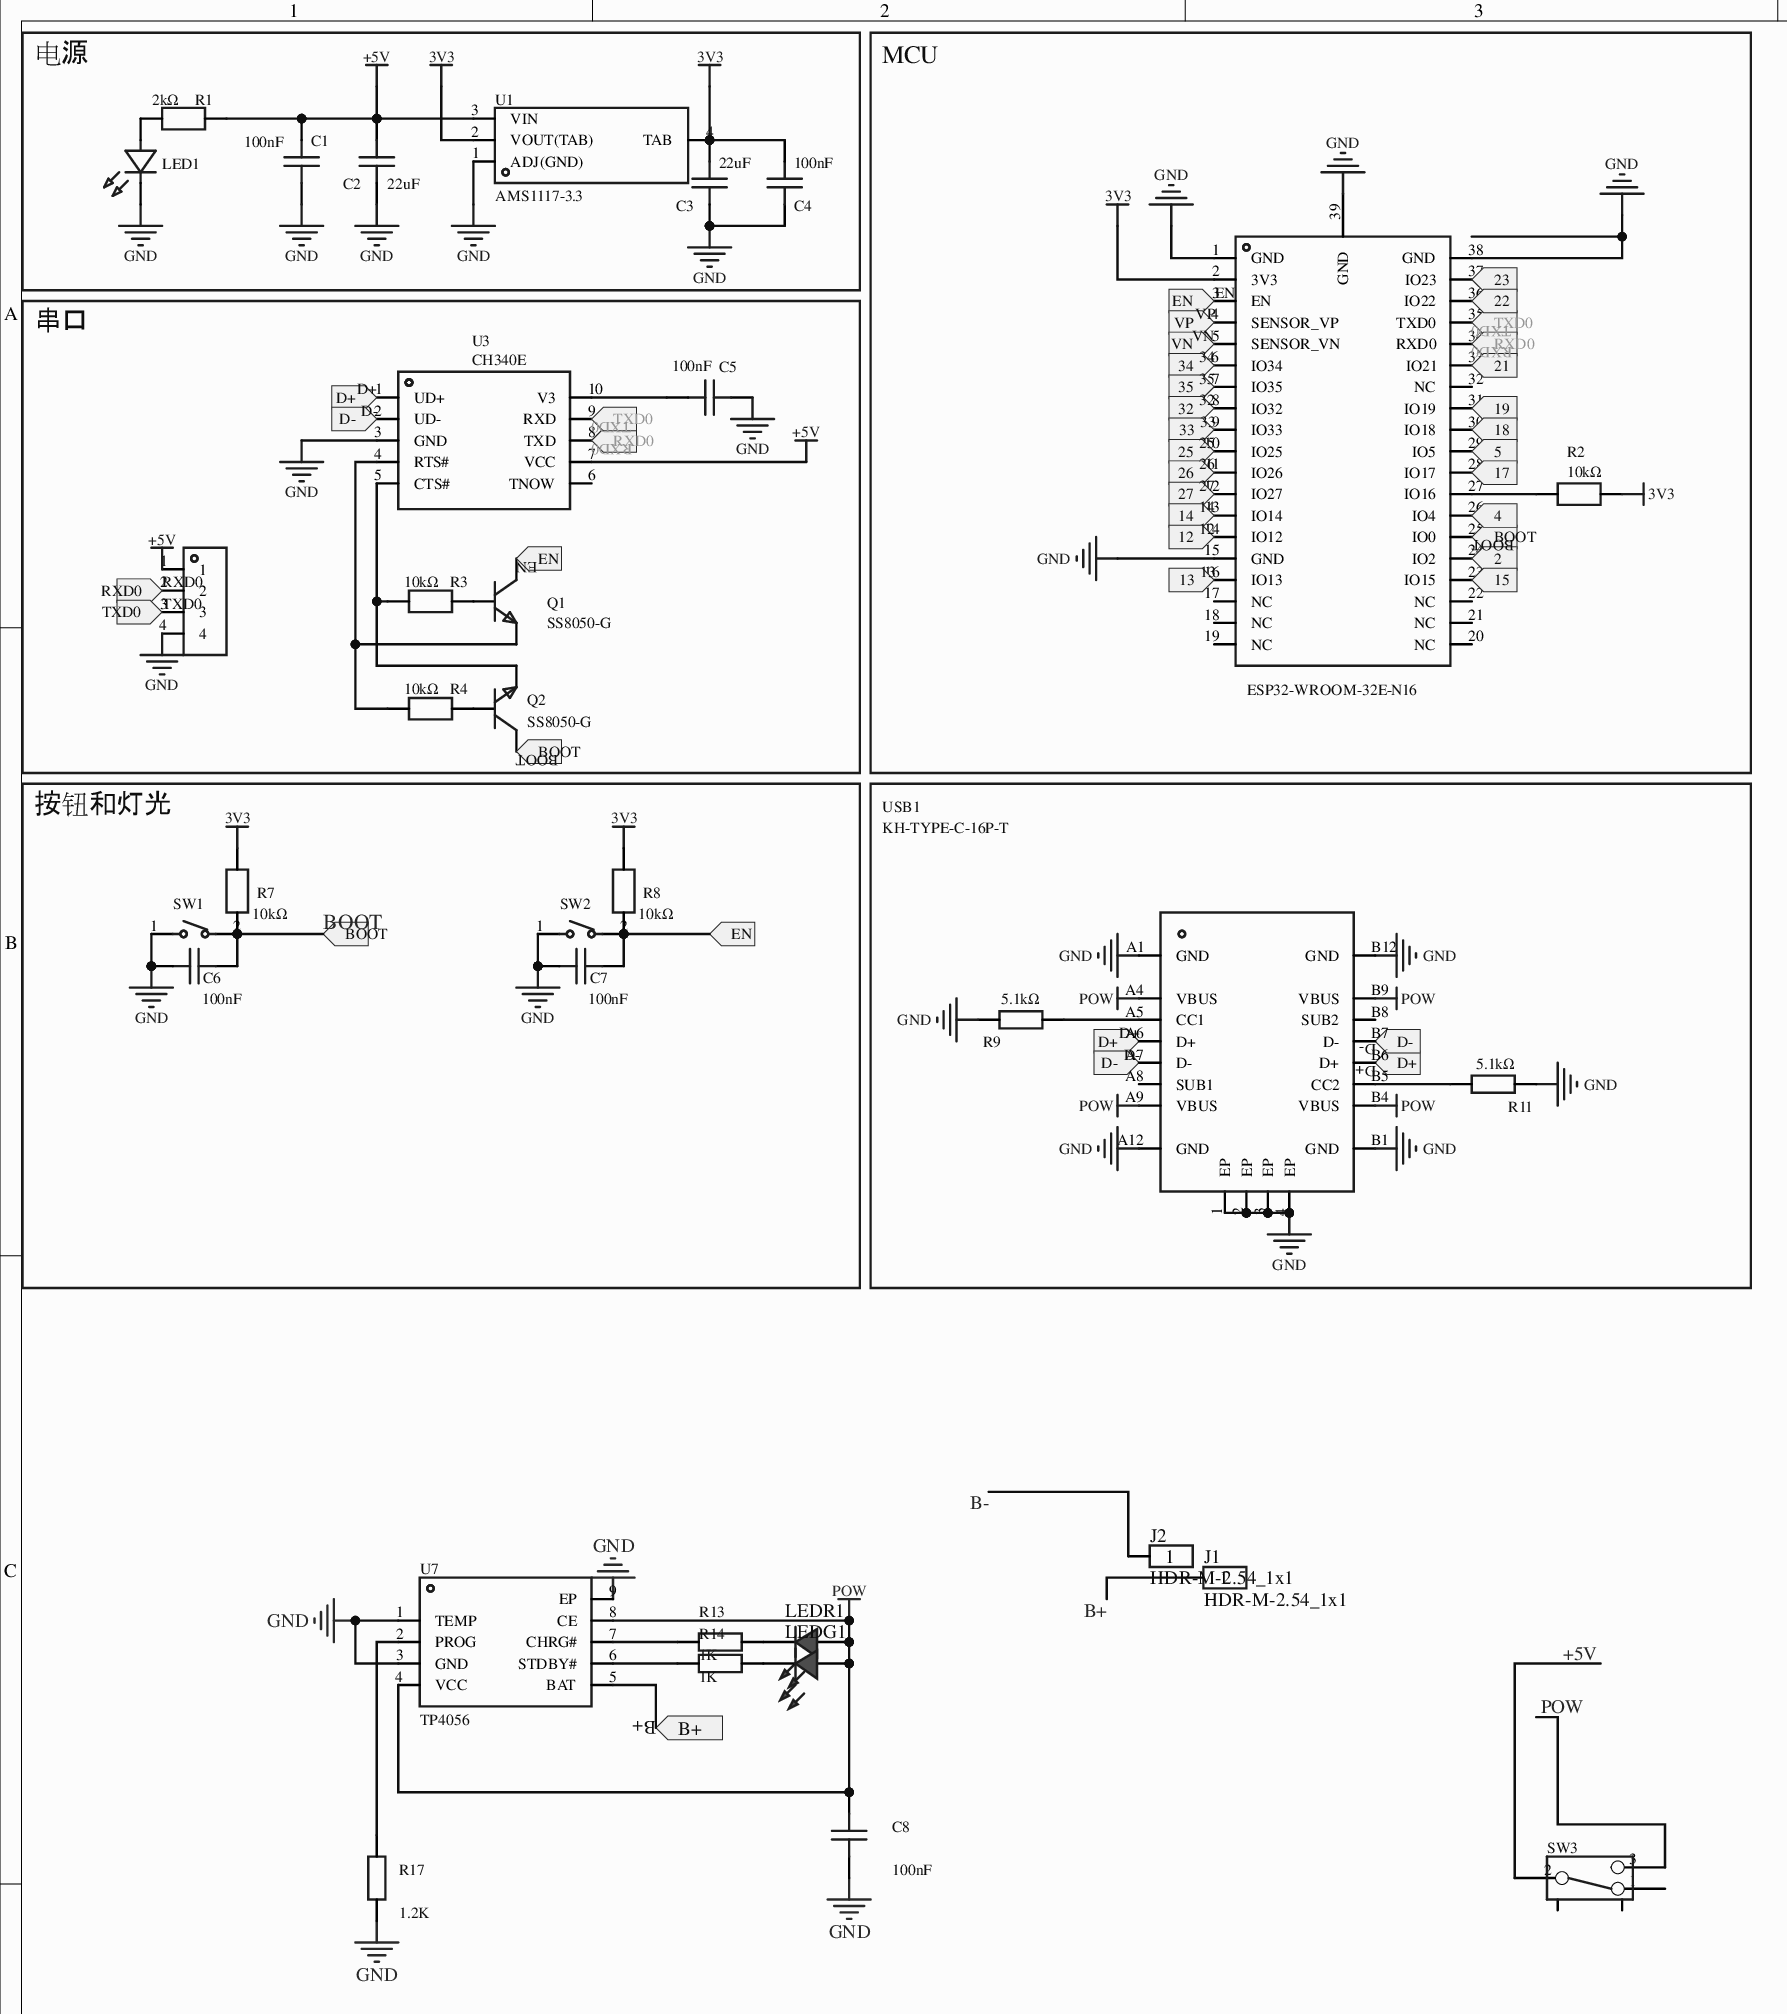
[diagram p0: MISC52063-3.schdoc]
# Altium project MISC52063-2.PrjPcb
1 sheet, 35 parts. Net scope: flat (ports and power ports of the same name join across sheets).
Board file: MISC52063.pcbdoc

## Sheet MISC52063-3.schdoc
size 420 x 297 mm; @Board Name: MISC52063; Version: V1.0; @Project Name: MISC52063; @Page Count: 1; @Update Date: 2026-03-21; @Create Date: 2026-03-21; @Schematic Name: MISC52063; @Page No: 0

### Parts
C1  100nF  [C0402]
C2  22uF  [C0603]
C3  22uF  [C0603]
C4  100nF  [C0402]
C5  100nF  [C0402]
C6  100nF  [C0402]
C7  100nF  [C0402]
C8  100nF  [C0603]
J1  HDR-M-2.54_1x1  [HDR-M-2.54_1X1]
J2  HDR-M-2.54_1x1  [HDR-M-2.54_1X1]
J3  2.54-1*4  [HDR-TH_4P-P2.54-V-M-1]  (value not drawn)
LED1  XL-1608SURC-06  [LED0603-RD_RED]  (value not drawn)
LEDG1  (no value)  [LED_0603]
LEDR1  (no value)  [LED_0603]
Q1  SS8050-G  [SOT-23-3_L2.9-W1.3-P1.90-LS2.4-BR]
Q2  SS8050-G  [SOT-23-3_L2.9-W1.3-P1.90-LS2.4-BR]
R1  2kΩ  [R0402]
R2  10kΩ  [R0402]
R3  10kΩ  [R0402]
R4  10kΩ  [R0402]
R7  10kΩ  [R0402]
R8  10kΩ  [R0402]
R9  5.1kΩ  [R0201]
R11  5.1kΩ  [R0201]
R13  1K  [R0603]
R14  1K  [R0603]
R17  1.2K  [R0603]
SW1  TSB008A2530A  [SW-SMD_L6.0-W3.5-LS8.0]  (value not drawn)
SW2  TSB008A2530A  [SW-SMD_L6.0-W3.5-LS8.0]  (value not drawn)
SW3  (no value)  [拨动开关_侧]
U1  AMS1117-3.3  [SOT-223-4_L6.5-W3.5-P2.30-LS7.0-BR]
U2  ESP32-WROOM-32E-N16  [WIFI-SMD_ESP32-WROOM-32E]
U3  CH340E  [MSOP-10_L3.0-W3.0-P0.50-LS5.0-BL]
U7  TP4056  [ESOP-8_L4.9-W3.9-P1.27-LS6.0-BL-EP]
USB1  KH-TYPE-C-16P-T  [USB-C-SMD_KH-TYPE-C-16P]

### Blocks framed on the sheet
电源: C1-C4 LED1 R1 U1
MCU: R2 U2
串口: C5 J3 Q1 Q2 R3 R4 U3
按钮和灯光: C6 C7 R7 R8 SW1 SW2

### Ports
2 (in), 4 (in), 5 (in), 12 (in), 13 (in), 14 (in), 15 (in), 17 (in), 18 (in), 19 (in), 21 (in), 22 (in), 23 (in), 25 (in), 26 (in), 27 (in), 32 (in), 33 (in), 34 (in), 35 (in), B+ (in), BOOT (in), D+ (in), D- (in), EN (in), RXD0 (in), TXD0 (in), VN (in), VP (in)

### Nets
3V3: C3.1 C4.2 R2.2 R7.1 R8.1 U1.2(VOUT(TAB)) U1.4(TAB) U2.2(3V3)
+5V: C1.2 C2.1 J3.1 R1.2 SW3.2 U1.3(VIN) U3.7(VCC)
GND: C1.1 C2.2 C3.2 C4.1 C5.1 C6.2 C7.2 C8.1 J3.4 LED1.1(K) R9.1 R11.2 R17.1 SW1.1 SW2.1 U1.1(ADJ(GND)) U2.1(GND) U2.15(GND) U2.38(GND) U2.39(GND) U3.3(GND) U7.1(TEMP) U7.3(GND) U7.9(EP) USB1.1(EP) USB1.2(EP) USB1.3(EP) USB1.4(EP) USB1.A1(GND) USB1.A12(GND) USB1.B1(GND) USB1.B12(GND)
POW: C8.2 LEDG1.2(A) LEDR1.2(A) SW3.3 U7.4(VCC) U7.8(CE) USB1.A4(VBUS) USB1.A9(VBUS) USB1.B4(VBUS) USB1.B9(VBUS)
12: U2.14(IO12) ; port 12
13: U2.16(IO13) ; port 13
14: U2.13(IO14) ; port 14
25: U2.10(IO25) ; port 25
26: U2.11(IO26) ; port 26
27: U2.12(IO27) ; port 27
32: U2.8(IO32) ; port 32
33: U2.9(IO33) ; port 33
34: U2.6(IO34) ; port 34
35: U2.7(IO35) ; port 35
B+: J1.1 U7.5(BAT) ; port B+
B-: J2.1
BOOT: C6.1 Q2.3(C) R7.2 SW1.2 U2.25(IO0) ; port BOOT
D+: U3.1(UD+) USB1.A6(D+) USB1.B6(D+) ; port D+
D-: U3.2(UD-) USB1.A7(D-) USB1.B7(D-) ; port D-
EN: C7.1 Q1.3(C) R8.2 SW2.2 U2.3(EN) ; port EN
RXD0: J3.2 U2.34(RXD0) U3.8(TXD) ; port RXD0
TXD0: J3.3 U2.35(TXD0) U3.9(RXD) ; port TXD0
VN: U2.5(SENSOR_VN) ; port VN
VP: U2.4(SENSOR_VP) ; port VP
NetC5_2: C5.2 U3.10(V3)
NetLED1_2: LED1.2(A) R1.1
NetLEDG1_1: LEDG1.1(C) R14.2
NetLEDR1_1: LEDR1.1(C) R13.2
NetQ1_1: Q1.1(B) R3.2
NetQ1_2: Q1.2(E) R4.1 U3.4(RTS#)
NetQ2_1: Q2.1(B) R4.2
NetQ2_2: Q2.2(E) R3.1 U3.5(CTS#)
NetR2_1: R2.1 U2.27(IO16)
NetR9_2: R9.2 USB1.A5(CC1)
NetR11_1: R11.1 USB1.B5(CC2)
NetR13_1: R13.1 U7.7(CHRG#)
NetR14_1: R14.1 U7.6(STDBY#)
NetR17_2: R17.2 U7.2(PROG)
NetU2_23: U2.23(IO15) ; port 15
NetU2_24: U2.24(IO2) ; port 2
NetU2_26: U2.26(IO4) ; port 4
NetU2_28: U2.28(IO17) ; port 17
NetU2_29: U2.29(IO5) ; port 5
NetU2_30: U2.30(IO18) ; port 18
NetU2_31: U2.31(IO19) ; port 19
NetU2_33: U2.33(IO21) ; port 21
NetU2_36: U2.36(IO22) ; port 22
NetU2_37: U2.37(IO23) ; port 23

Not connected (* = marked no-connect by the designer): SW3 1 4 5; U2 17(NC)* 18(NC)* 19(NC)* 20(NC)* 21(NC)* 22(NC)* 32(NC)*; U3 6(TNOW)*; USB1 A8(SUB1)* B8(SUB2)*

### Library data of the parts
C1 C4-C7 = C1005X5R104METS: 容值:100nF;精度:±20%;额定电压:16V;材质(温度系数):X5R;; Manufacturer: DARFON(达方); Origin Footprint: C0603; Convert to PCB: yes; Check: true; ModelId: 36a51122f27c49738f86b3bfa98863e0; ModelName: C0402_L1.0-W0.5-H0.5; ModelTransform: 39.37,19.685,0,0,0,0,0,0,0; Tolerance: ±20%; Voltage Rated: 16V; Temperature Coefficient: X5R; Device: C1005X5R104METS; Symbol: C1005X5R104METS; Supplier Part: C147680; Supplier: LCSC; Manufacturer Part: C1005X5R104METS; Add into BOM: yes; LCSC Part Name: 100nF ±20% 16V; Supplier Footprint: 0402; JLCPCB Part Class: Extended Part; Datasheet: https://atta.szlcsc.com/upload/public/pdf/source/20190902/C424339_65E80B11205B7B8B44D3E281FEB76198.pdf; FootprintName: C0402; Value: 100nF
C2 C3 = HGC0603R5226M100NTHJ: 容值:22uF;精度:±20%;额定电压:10V;材质(温度系数):X5R;; Manufacturer: Chinocera(华瓷); Convert to PCB: yes; Check: true; ModelId: ac125912035d415993ca9572d50418b1; ModelName: C0603_L1.6-W0.8-H0.8; ModelTransform: 62.992,31.496,0,0,0,0,0,0,0; Tolerance: ±20%; Voltage Rated: 10V; Temperature Coefficient: X5R; Origin Footprint: C0603; Device: HGC0603R5226M100NTHJ; Symbol: HGC0603R5226M100NTHJ; Supplier Part: C7432770; Supplier: LCSC; Manufacturer Part: HGC0603R5226M100NTHJ; Add into BOM: yes; LCSC Part Name: 22uF ±20% 10V; Supplier Footprint: 0603; JLCPCB Part Class: Extended Part; Datasheet: https://atta.szlcsc.com/upload/public/pdf/source/20240320/FAC3FEC40A78BC5CCCE96C232A94D860.pdf; FootprintName: C0603; Value: 22uF
C8 = CAP_0603: Symbol: CapAcitance; 3D Model: ac125912035d415993ca9572d50418b1; 3D Model Transform: 62.992,31.496,0,0,0,0,0,0,0; ConvertToPcb: yes; ModelName: C0603_L1.6-W0.8-H0.8; Device: CAP_0603; Value: 100nF; Supplier Footprint: 0603; AddInBom: yes; FootprintName: C0603
J1 J2 = HDR-M-2.54_1x1: Add into BOM: yes; 3D Model Transform: 100,100,0,0,0,0,0,0,-118.11; 3D Model: 9821adf8e7254e65b824f7d81520e51f; Symbol: HDR-M-2.54_1x1; Device: HDR-M-2.54_1x1; Convert to PCB: yes; Supplier Part: C81276; Supplier: LCSC; Origin 3D Model Title: HDR-M-2.54_1x1; FootprintName: HDR-M-2.54_1X1; ModelName: HDR-M-2.54_1x1
J3 = 2.54-1*4: 插针结构:1x4P;间距:2.54mm;排数:单排;总PIN位数:4P;; Manufacturer: ZHOURI(洲日); Origin Footprint: HDR-M-2.54_1X4; Convert to PCB: yes; Check: true; ModelId: f8e5d153169943fabcf3383e1c9553c6; ModelTransform: 399.999,100,0,0,0,0,0,0,-118.11; Pin Structure: 1x4P; Pitch: 2.54mm; Device: 2.54-1*4; Symbol: 2.54-1*4; Supplier Part: C5116483; Supplier: LCSC; Manufacturer Part: 2.54-1*4; Add into BOM: yes; LCSC Part Name: 2.54-1*4; Supplier Footprint: 插件,P=2.54mm; JLCPCB Part Class: Extended Part; Datasheet: https://atta.szlcsc.com/upload/public/pdf/source/20220729/BC3442D33C9CDBB7F5DC20B12A8605A8.pdf; FootprintName: HDR-TH_4P-P2.54-V-M-1; ModelName: HDR-M-2.54_1x4; Number of Rows: 单排; Number of Pins: 4P
LED1 = XL-1608SURC-06: 发光颜色:红色;功率:55mW;正向电流:25mA;主波长:617nm~621nm;透镜颜色:无色透明透镜;色温:-;发光角度:120°;载带方式:正贴;工作温度:-30℃~+85℃;; Manufacturer: XINGLIGHT(成兴光); AddInBom: yes; ModelId: 74041d3a270d435c8600a9ab9b7641c0; ModelTransform: 63.7794,31.496,0,0,0,0,0,0,0; Emitted Color: 红色; Power Dissipation: 55mW; Forward Current: 25mA; Peak Wavelength: 623nm; Lens Color: 无色透明透镜; Viewing Angle: 120°; Mounting Sytle: 正贴; Symbol: XL-1608SURC-06; Device: XL-1608SURC-06; LCSC Part Name: XL-1608SURC-06; SupplierPart: C965799; ManufacturerPart: XL-1608SURC-06; Supplier Footprint: 0603; JLCPCB Part Class: Extended Part; Datasheet: https://atta.szlcsc.com/upload/public/pdf/source/20221102/D860AFDD1CDB02C5A8064103A32707E2.pdf; Supplier: LCSC; ConvertToPcb: yes; FootprintName: LED0603-RD_RED; ModelName: LED0603-RD_RED; Dominant Wavelength: 617nm~621nm; Color Temperature: -; Operating Temperature: -30℃~+85℃
LEDG1 LEDR1 = LED_0603-R: Symbol: LED_R; Convert to PCB: yes; 3D Model: dd8257b0d61a4cd7b68939a056e08095; 3D Model Transform: 58.72,29.4,22.03,0,0,0,0,0,0; ModelName: LED-0603_R; Device: LED_0603-R; Add into BOM: yes; Supplier Footprint: 0603; FootprintName: LED_0603
Q1 Q2 = SS8050-G: 晶体管类型:NPN;集电极电流(Ic):1.5A;集射极击穿电压(Vceo):25V;功率(Pd):300mW;直流电流增益(hFE@Ic,Vce):200@100mA,1V;; Manufacturer: CJ(江苏长电/长晶); Symbol: SS8050-G_C164885; Convert to PCB: yes; Check: true; ModelId: c62791f0466c4ae2a892c056b845b0ca; ModelName: SOT-23-3P_L2.9-W1.3-H1.0-LS2.4-P0.95; ModelTransform: 98.425,114.173,0,180,0,0,0.0005,-0.0005,0; Transistor Type: NPN; Collector Current (Ic): 1.5A; Collector-Emitter Breakdown Voltage (Vceo): 25V; Power Dissipation (Pd): 300mW; Transition Frequency (fT): 100MHz; Collector Cut-Off Current (Icbo): 100nA; Collector-Emitter Saturation Voltage (VCE(sat)@Ic,Ib): 500mV@800mA,80mA; Origin Footprint: SOT-23-3_L2.9-W1.3-P1.90-LS2.4-BR; Device: SS8050-G; Supplier: LCSC; Manufacturer Part: SS8050-G; Supplier Part: C164885; JLCPCB Part Class: Extended Part; Add into BOM: yes; LCSC Part Name: SS8050-G(RANGE:200-350) H档(200-350); Supplier Footprint: SOT-23; Datasheet: https://atta.szlcsc.com/upload/public/pdf/source/20180130/C177739_15172974524031323483.pdf; FootprintName: SOT-23-3_L2.9-W1.3-P1.90-LS2.4-BR; DC Current Gain (hFE@Ic,Vce): 200@100mA,1V; Operating Temperature: -
R1 = SC0402F2001F2ANRH: 阻值:2kΩ;精度:±1%;功率:-;温度系数:±100ppm/℃;; Manufacturer: Sunway(信维通信); Convert to PCB: yes; ModelId: 671aefced39d4c318694bba8bd8efd39; ModelName: R0402_L1.0-W0.5-H0.5; ModelTransform: 39.37,19.685,0,0,0,0,0,0.0005,0; Tolerance: ±1%; Device: SC0402F2001F2ANRH; Symbol: SC0402F2001F2ANRH; Supplier Part: C3152076; Supplier: LCSC; Manufacturer Part: SC0402F2001F2ANRH; Add into BOM: yes; LCSC Part Name: 2kΩ ±1%; Supplier Footprint: 0402; JLCPCB Part Class: Extended Part; Datasheet: https://atta.szlcsc.com/upload/public/pdf/source/20220728/FFCE43BB6DF8FA16AEE331F0F4B289DE.pdf; FootprintName: R0402; Value: 2kΩ; Power(Watts): -; Temperature Coefficient: ±100ppm/℃
R2-R4 R7 R8 = RCA0210KJLF: 阻值:10kΩ;精度:±5%;功率:62.5mW;; Manufacturer: HKR(香港电阻); Overload Voltage (Max): 75V; Temperature Coefficient: ±100ppm/℃; Origin Footprint: R0603; Convert to PCB: yes; Check: true; ModelId: 671aefced39d4c318694bba8bd8efd39; ModelName: R0402_L1.0-W0.5-H0.5; ModelTransform: 39.37,19.685,0,0,0,0,0,0.0005,0; Tolerance: ±5%; Power(Watts): 62.5mW; Type: 厚膜电阻; Operating Temperature Range: -55℃~+155℃; Device: RCA0210KJLF; Symbol: RCA0210KJLF; Supplier Part: C22356213; Supplier: LCSC; Manufacturer Part: RCA0210KJLF; Add into BOM: yes; LCSC Part Name: 10kΩ ±5% 62.5mW; Supplier Footprint: 0402; JLCPCB Part Class: Extended Part; Datasheet: https://atta.szlcsc.com/upload/public/pdf/source/20240312/EB29F8B3E9AD4CE07E65E9956C47F4F5.pdf; FootprintName: R0402; Value: 10kΩ
R9 R11 = RTT01512JTH: 阻值:5.1kΩ;精度:±5%;功率:50mW;温度系数:±200ppm/℃;; Manufacturer: RALEC(旺诠); Overload Voltage (Max): 75V; Origin Footprint: R0603; Convert to PCB: yes; Check: true; ModelId: 0e006ba4c37b4b73b0e85d5d1c6800cb; ModelName: R0201_L0.6-W0.3-H0.3; ModelTransform: 23.622,11.811,0,0,0,0,0,-0.0005,0; Tolerance: ±5%; Power(Watts): 50mW; JLCPCB Part Class: Extended Part; Type: 厚膜电阻; Value: 5.1kΩ; Operating Temperature Range: -55℃~+155℃; Device: RTT01512JTH; Symbol: RTT01512JTH; Supplier Part: C158467; Supplier: LCSC; Manufacturer Part: RTT01512JTH; Add into BOM: yes; LCSC Part Name: 5.1kΩ ±5% 50mW; Supplier Footprint: 0201; Datasheet: https://atta.szlcsc.com/upload/public/pdf/source/20191219/C158410_884373A5B7E1BC76BF57BC45A946C093.pdf; FootprintName: R0201; Temperature Coefficient: ±200ppm/℃
R13 R14 R17 = Res_0603: Symbol: 电阻; 3D Model: fc143cca1e79419f9cd78b61e9279f08; 3D Model Transform: 31.8897,63.7794,0,90,0,0,0,0,0; ConvertToPcb: yes; Device: Res_0603; Supplier Footprint: 0603; AddInBom: yes; FootprintName: R0603; ModelName: R0603
  R13 R14: Value: 1K
  R17: Value: 1.2K
SW1 = TSB008A2530A: 按钮形状:矩形按钮;作用力:3N;安装方式:立贴;开关长度:6mm;开关宽度:3.5mm;开关高度:2.5mm;触点电流:50mA;额定电压(AC):-;额定电压(DC):12V;机械寿命:-;; Manufacturer: BZCN(博众电气); Circuit: 单刀单掷; Insulation Resistance: 100MΩ; Origin Footprint: KEY-SMD_2P-L6.2-W3.6-LS8.0; 制造商: 韩国韩荣; Convert to PCB: yes; Check: true; ModelId: 5140287d81af41d993b04546ae6cc4e8; ModelName: SW-SMD_L6.0-W3.5-H5.0-P7.5-LS8.0; ModelTransform: 314.96,137.795,0,0,0,0,0,0,0; Actuator Style: 矩形按钮; Operating Force: 3N; Switch Length: 6mm; Switch Width: 3.5mm; Switch Height: 2.5mm; Contact Current: 50mA; Voltage Rating (DC): 12V; Actuator/Cap Color: 白色; With Lamp: -; Operating Temperature: -25℃~+85℃; Device: TSB008A2530A; Symbol: TSB008A2530A; Supplier Part: C2888954; Supplier: LCSC; Manufacturer Part: TSB008A2530A; Add into BOM: yes; LCSC Part Name: 6*3.5*2.5mm 立贴 轻触开关; Supplier Footprint: SMD; JLCPCB Part Class: Extended Part; Datasheet: https://atta.szlcsc.com/upload/public/pdf/source/20210906/C2888955_77EE870C858B4B9378E660F9B12998D5.pdf; FootprintName: SW-SMD_L6.0-W3.5-LS8.0; Mounting Style: 立贴; Voltage Rating (AC): -; Mechanical Life: -
SW2 = TSB008A2530A: 按钮形状:矩形按钮;作用力:3N;安装方式:立贴;开关长度:6mm;开关宽度:3.5mm;开关高度:2.5mm;触点电流:50mA;额定电压(AC):-;额定电压(DC):12V;机械寿命:-;; Manufacturer: BZCN(博众电气); AddInBom: yes; ModelId: 5140287d81af41d993b04546ae6cc4e8; ModelName: SW-SMD_L6.0-W3.5-H5.0-P7.5-LS8.0; ModelTransform: 314.96,137.795,0,0,0,0,0,0,0; Actuator Style: 矩形按钮; Operating Force: 3N; Switch Length: 6mm; Switch Width: 3.5mm; Switch Height: 2.5mm; Contact Current: 50mA; Voltage Rating (DC): 12V; Actuator/Cap Color: 白色; Symbol: TSB008A2530A; Device: TSB008A2530A; LCSC Part Name: 6*3.5*2.5mm 立贴 轻触开关; SupplierPart: C2888954; ManufacturerPart: TSB008A2530A; Supplier Footprint: SMD; JLCPCB Part Class: Extended Part; Datasheet: https://atta.szlcsc.com/upload/public/pdf/source/20210906/C2888955_77EE870C858B4B9378E660F9B12998D5.pdf; Supplier: LCSC; ConvertToPcb: yes; FootprintName: SW-SMD_L6.0-W3.5-LS8.0; Mounting Style: 立贴; Voltage Rating (AC): -; Mechanical Life: -
SW3 = 拨动开关_侧: Symbol: 拨动开关; ConvertToPcb: yes; ModelId: 10ea2cc5ba004a75b38812aadef1031f0819f05c4eef4c71ace90d822a990e87; ModelName: SW-TH_SK-12D07-VG3; ModelTransform: 337.98,287.46,295.24,0,0,0,0,-57,-110; Device: 拨动开关_侧; AddInBom: yes; Supplier Footprint: 插件; FootprintName: 拨动开关_侧
U1 = AMS1117-3.3_C347222: 输出类型:固定;最大输入电压:12V;输出电压:3.3V;最大输出电流:1A;电源纹波抑制比(PSRR):60dB@(120Hz);输出极性:正极;; Manufacturer: UMW(友台半导体); Origin Footprint: SOT-223-3_L6.5-W3.4-P2.30-LS7.0-BR; Convert to PCB: yes; Check: true; ModelId: 925194bf9823436183a3e0b978a8d076; ModelName: SOT-223-4P_L6.5-W3.5-H1.6-LS7.0-P2.30; ModelTransform: 279.89794,255.905,0,180,0,0,-0.0005,-0.0005,0; Output Type: 固定; Maximum Input Voltage: 12V; Output Voltage: 3.3V; MAX Output Current: 1A; Dropout Voltage: 1.3V@(1A); Output Polarity: 正极; Number of Outputs: 1; Device: AMS1117-3.3_C347222; Symbol: AMS1117-3.3_C347222; Supplier: LCSC; Manufacturer Part: AMS1117-3.3; Supplier Part: C347222; JLCPCB Part Class: Extended Part; Add into BOM: yes; LCSC Part Name: 输出:3.3V 电流:1A 耐压:12V; Supplier Footprint: SOT-223; Datasheet: https://atta.szlcsc.com/upload/public/pdf/source/20231109/155D79A26D9DB04352555A58D5969DC8.pdf; FootprintName: SOT-223-4_L6.5-W3.5-P2.30-LS7.0-BR; Power Supply Rejection Ratio (PSRR): 60dB@(120Hz); standby current: -; Noise: -; Feature: -; Operating Temperature: -
U2 = ESP32-WROOM-32E-N16_C701343: ESP32-WROOM-32E 集成 ESP32-D0WD-V3 芯片，具有高稳定性和安全性能。; Manufacturer: ESPRESSIF(乐鑫); Origin Footprint: WIFI-SMD_ESP32-WROOM-32E-A; Symbol: ESP32-WROOM-32E(16MB); Convert to PCB: yes; Check: true; ModelId: 002cfca93c884bd0a0e44ace4f3b2041; ModelName: WIFI-SMD_L25.5-W18.0-H3.1-ESP32-WROOM-32E; ModelTransform: 1003.935,708.66,0,180,0,0,-148.762,0,0; Device: ESP32-WROOM-32E-N16_C701343; Supplier: LCSC; Supplier Part: C701343; Manufacturer Part: ESP32-WROOM-32E-N16; JLCPCB Part Class: Extended Part; Add into BOM: yes; LCSC Part Name: 通用型Wi-Fi+BT+BLE MCU模组; Supplier Footprint: SMD,18x25.5mm; Datasheet: https://atta.szlcsc.com/upload/public/pdf/source/20200730/C701341_95E089979D39CD8D2471FDC7C7AF29A1.pdf; FootprintName: WIFI-SMD_ESP32-WROOM-32E
U3 = CH340E: 应用功能:收发器;接口协议:USB 2.0;数据速率:2Mbps;; Manufacturer: WCH(南京沁恒); Convert to PCB: yes; Check: true; ModelId: b42a31f9e1fa4643bc7ea573b9bba7ed; ModelName: MSOP-10_L3.0-W3.0-H1.1-LS5.0-P0.50; ModelTransform: 118.11,196.85,0,0,0,0,0,0,0; Applications Function: 收发器; Protocol: USB 2.0; Supply Voltage: 3.3V；5V; Data Rate: 2Mbps; Origin Footprint: MSOP-10_L3.0-W3.0-P0.50-LS5.0-BL; Device: CH340E; Symbol: CH340E; Supplier: LCSC; Manufacturer Part: CH340E; Supplier Part: C99652; JLCPCB Part Class: Extended Part; Add into BOM: yes; LCSC Part Name: USB转串口芯片 CH340; Supplier Footprint: MSOP-10; Datasheet: https://atta.szlcsc.com/upload/public/pdf/source/20230530/6E401E9554E9F5311886CC8B3F89B62E.pdf; FootprintName: MSOP-10_L3.0-W3.0-P0.50-LS5.0-BL
U7 = TP4056_C725790: Manufacturer: UMW(友台半导体); 3D Model: d3e00daa36c445139c055a3b9efb85d2; 3D Model Transform: 240.157,192.913,0,90,0,0,0,0,0; AddInBom: yes; ModelName: ESOP-8_L4.9-W3.9-H1.6-LS6.0-P1.27; Symbol: TP4056_C725790; Device: TP4056_C725790; LCSC Part Name: TP4056; Supplier Part: C725790; Manufacturer Part: TP4056; Supplier Footprint: ESOP-8; JLCPCB Part Class: Extended Part; Datasheet: https://atta.szlcsc.com/upload/public/pdf/source/20211011/37515E71BA298E23D23475482C49633D.pdf; Supplier: LCSC; ConvertToPcb: yes; FootprintName: ESOP-8_L4.9-W3.9-P1.27-LS6.0-BL-EP
USB1 = KH-TYPE-C-16P-T: 连接器类型:Type-C;标准:-;公母:母;端口数量:1;触点数量:16P;安装方式:卧贴;额定电流 - 电源:500mA;工作温度范围:-30℃~+80℃;; Manufacturer: kinghelm(金航标); Convert to PCB: yes; Check: true; ModelId: f2c381012fbf47e0b76dea5162270f01; ModelTransform: 351.9678,307.48,0,0,0,0,0,-45.275,-43.307; Connector Type: Type-C; Gender: 母; Number of Ports: 1; Number of Contacts: 16P; Current Rating - Power (Max): 500mA; Origin Footprint: USB-C-SMD_KH-TYPE-C-16P; Device: KH-TYPE-C-16P-T; Symbol: KH-TYPE-C-16P-T; Supplier: LCSC; Supplier Part: C709358; Manufacturer Part: KH-TYPE-C-16P-T; JLCPCB Part Class: Extended Part; Add into BOM: yes; LCSC Part Name: Type-C 母 卧贴; Supplier Footprint: SMD; Datasheet: https://atta.szlcsc.com/upload/public/pdf/source/20200722/C709358_5A99A991362FD50EC94EB58A838F95BB.pdf; FootprintName: USB-C-SMD_KH-TYPE-C-16P; ModelName: USB-C-SMD_KH-TYPE-C-16P; Standard: -; Mounting Style: 卧贴; Operating Temperature Range: -30℃~+80℃